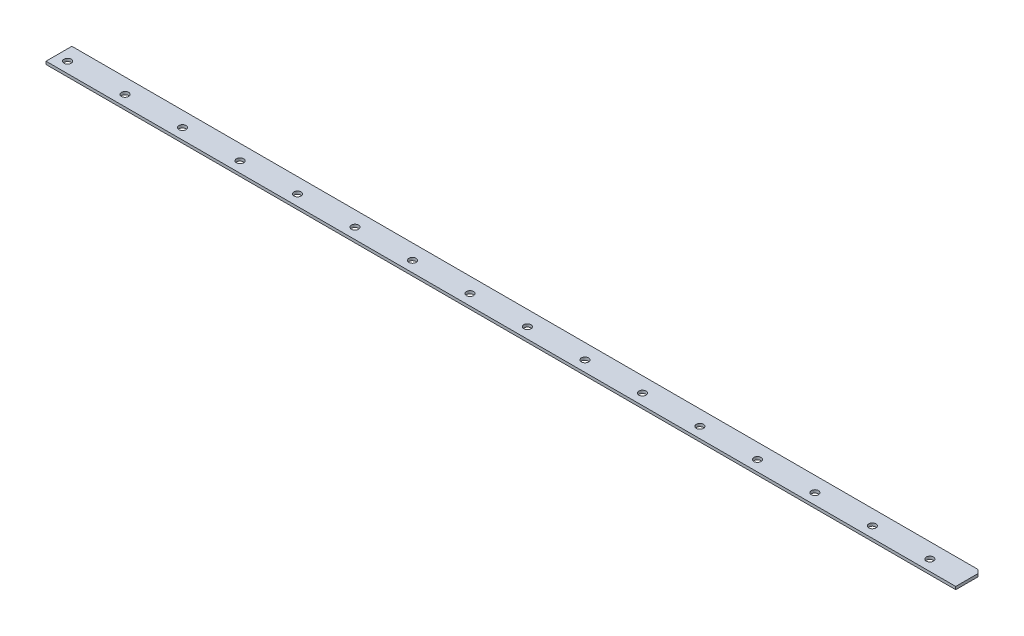
SolidWorks part; units mm, degrees
material "Q235"
ref_plane "前视基准面" through (0, 0, 0) normal (0, 0, 1) x (1, 0, 0)
ref_plane "上视基准面" through (0, 0, 0) normal (0, 1, 0) x (1, 0, 0)
ref_plane "右视基准面" through (0, 0, 0) normal (1, 0, 0) x (0, 0, -1)
sketch "草图1" plane through (0, 0, 0) normal (0, 1, 0) x (1, 0, 0)
  line L0 (-2.2, 0) -> (2.2, 0) construction
  line L1 (-1266, 0) -> (0, 0)
  line L2 (-1266, 0) -> (-1266, -36)
  line L3 (-1266, -36) -> (0, -36)
  line L4 (0, 0) -> (0, -36)
  line L5 (0, -2.2) -> (0, 2.2) construction
  dimension "D1" = 36
  dimension "D2" = 1266
extrude "凸台-拉伸1" add sketch "草图1" along normal blind 4
chamfer "倒角1" distance 5 angle 45 1 edges at (0, 2, 0)
hole_wizard "Ø10.0 (10) 直径孔1" positions "草图4" profile "草图3" hole size "Ø10.0" standard "GB" end condition through all
sketch "草图4" plane through (0, 4, 0) normal (0, 1, 0) x (-1, 0, 0)
  line L0 (1266, 36) -> (0, 36) construction
  line L2 (1266, 0) -> (1266, 36) construction
  point P0 (1251, 21)
  dimension "D1" = 15
  dimension "D2" = 15
sketch "草图3" plane through (-1251, 4, 21) normal (1, 0, 0) x (0, 0, 1)
  line L0 (0, 0) -> (0, 4)
  line L1 (0, 4) -> (5, 4)
  line L2 (5, 4) -> (5, 0)
  line L5 (5, 0) -> (0, 0)
  line L11 (0, -6.35) -> (0, 107.95) construction
  dimension "通孔孔直径" = 10
  dimension "通孔孔深度" = 4
pattern_linear "阵列(线性)1" count 16 spacing 80 along (1, 0, 0) of "Ø10.0 (10) 直径孔1"
